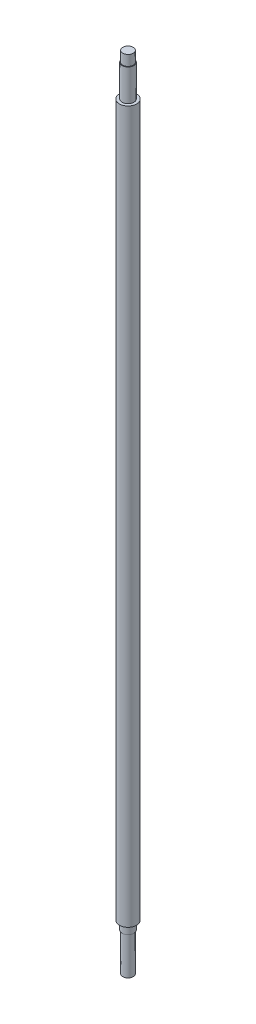
from build123d import *


with BuildPart() as part:
    # Sketch2 → Revolve1 (revolve)
    with BuildSketch(Plane.XY, mode=Mode.PRIVATE) as revolve1_sk:
        Polygon((0, 0), (7.5, 0), (7.5, -15), (8.5, -15), (8.5, -61), (12.5, -61), (12.5, -1090), (8.5, -1090), (8.5, -1102), (7.5, -1102), (7.5, -1157), (0, -1157), align=None)
    revolve(revolve1_sk.sketch.rotate(Axis((0, 0, 0), (0, 1, 0)), 90), axis=Axis((0, 0, 0), (0, 1, 0)))


solid = part.part
